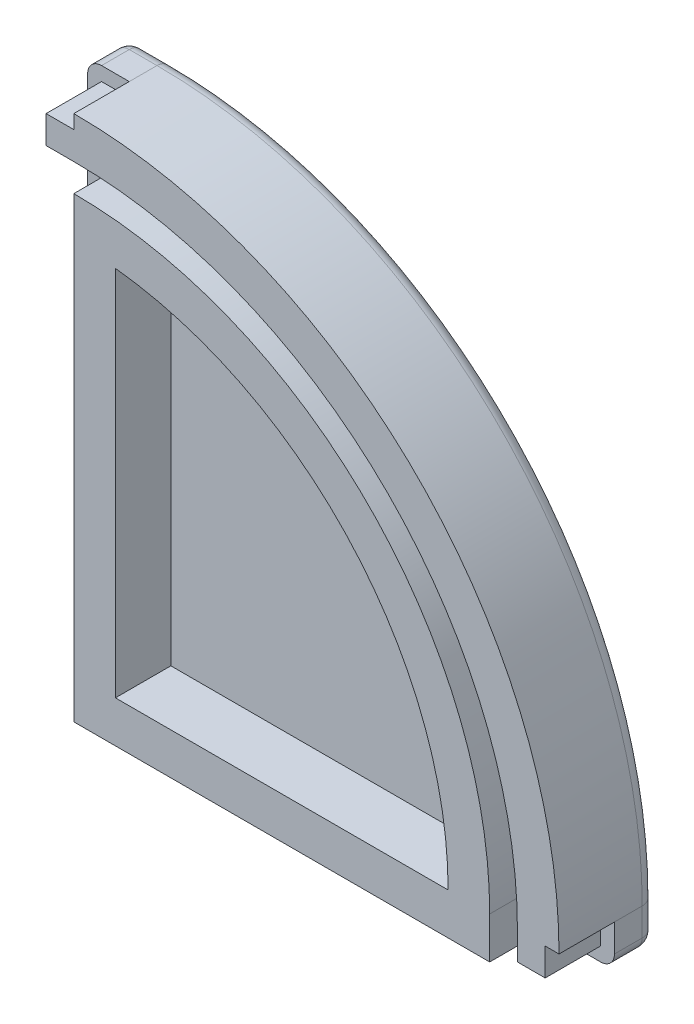
SolidWorks part; units mm, degrees
ref_plane "Frontal" through (0, 0, 0) normal (0, 0, 1) x (1, 0, 0)
ref_plane "Superior" through (0, 0, 0) normal (0, 1, 0) x (1, 0, 0)
ref_plane "Direito" through (0, 0, 0) normal (1, 0, 0) x (0, 0, -1)
sketch "Sketch1" plane through (0, 0, 0) normal (0, 0, 1) x (1, 0, 0)
  line L0 (0, 0) -> (0, 19)
  line L1 (19, 0) -> (0, 0)
  line L2 (0, 19) -> (1.5, 19)
  line L3 (19, 1.5) -> (19, 0)
  arc A0 (1.5, 19) -> (19, 1.5) centre (1.5, 1.5) cw
  dimension "D1" = 19
  dimension "D2" = 1.5
  dimension "D3" = 1.5
extrude "Boss-Extrude1" add sketch "Sketch1" along normal blind 1.5
sketch "Sketch2" plane through (0, 0, 1.5) normal (0, 0, 1) x (1, 0, 0)
  line L0 (1.5, 19) -> (1.5, 18.5)
  line L1 (1.5, 18.5) -> (0.5, 18.5)
  line L2 (0.5, 18.5) -> (0.5, 17.5)
  line L3 (0.5, 17.5) -> (1.5, 17.5)
  line L4 (17.5, 1.5) -> (17.5, 0.5)
  line L5 (17.5, 0.5) -> (18.5, 0.5)
  line L6 (18.5, 0.5) -> (18.5, 1.5)
  line L7 (18.5, 1.5) -> (19, 1.5)
  line L8 (1.5, 16.5) -> (1.5, 0)
  line L9 (0, 0) -> (19, 0) construction
  line L11 (1.5, 0) -> (16.5, 0)
  line L13 (16.5, 0) -> (16.5, 1.5)
  line L14 (3, 14.9164) -> (3, 1.5)
  line L15 (3, 1.5) -> (15, 1.5)
  line L16 (15, 1.5) -> (15, 1.5)
  line L17 (0, 19) -> (0, 0) construction
  line L18 (1.5, 19) -> (0, 19) construction
  line L19 (19, 0) -> (19, 1.5) construction
  arc A0 (1.5, 17.5) -> (17.5, 1.5) centre (1.5, 1.5) cw
  arc A1 (19, 1.5) -> (1.5, 19) centre (1.5, 1.5) ccw
  arc A2 (16.5, 1.5) -> (1.5, 16.5) centre (1.5, 1.5) ccw
  arc A3 (15, 1.5) -> (3, 14.9164) centre (1.5, 1.5) ccw
  dimension "D6" = 16
  dimension "D10" = 13.5
  dimension "D2" = 1.5
  dimension "D3" = 0.5
  dimension "D4" = 0.5
  dimension "D5" = 1
  dimension "D7" = 1
  dimension "D8" = 0.5
  dimension "D9" = 1
  dimension "D11" = 1
  dimension "D12" = 16.5
  dimension "D1" = 1.5
extrude "Boss-Extrude2" add sketch "Sketch2" along normal blind 2
fillet "Filete1" radius 0.5 7 edges at (19, 0.75, 0) (0.75, 19, 0) (19, 0, 0.75) (0, 19, 0.75) (0, 9.5, 0) (9.5, 0, 0) (13.8744, 13.8744, 0)
